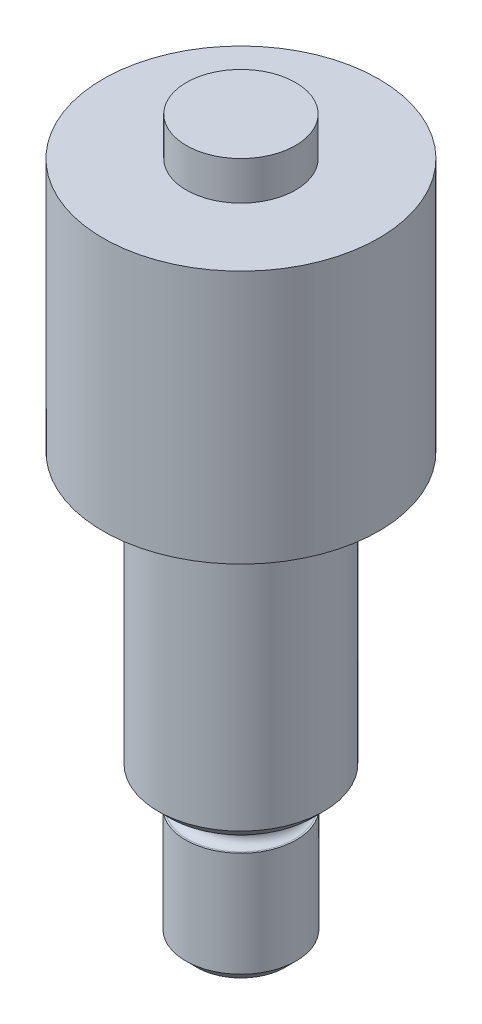
SolidWorks part; units mm, degrees
material "35"
ref_plane "前视基准面" through (0, 0, 0) normal (0, 0, 1) x (1, 0, 0)
ref_plane "上视基准面" through (0, 0, 0) normal (0, 1, 0) x (1, 0, 0)
ref_plane "右视基准面" through (0, 0, 0) normal (1, 0, 0) x (0, 0, -1)
sketch "草图1" plane through (0, 0, 0) normal (0, 0, 1) x (1, 0, 0)
  line L0 (0, 0) -> (9.9, 0)
  line L1 (9.9, 0) -> (9.9, -7)
  line L2 (9.9, -7) -> (25, -7)
  line L3 (25, -7) -> (25, -53)
  line L4 (25, -53) -> (15, -53)
  line L5 (15, -53) -> (15, -104)
  line L6 (15, -104) -> (8.2, -104)
  line L7 (8.2, -104) -> (8.2, -109)
  line L8 (8.2, -109) -> (10, -109)
  line L9 (10, -109) -> (10, -130)
  line L10 (10, -130) -> (0, -130)
  line L13 (0, -130) -> (0, 0)
  dimension "D1" = 9.9
  dimension "D2" = 7
  dimension "D3" = 46
  dimension "D4" = 5
  dimension "D5" = 130
  dimension "D7" = 25
  dimension "D8" = 15
  dimension "D9" = 8.2
  dimension "D11" = 10
  dimension "D12" = 51
revolve "旋转1" add sketch "草图1" angle 360 about L13
cosmetic thread "装饰螺纹线1" parameters "D2"=17.294
chamfer "倒角1" distance 2 angle 45 2 edges at (0, -104, -15) (0, -130, -10)
fillet "圆角1" radius 1 1 edges at (0, -53, -15)
fillet "圆角2" radius 1.5 2 edges at (0, -104, -8.2) (0, -109, -8.2)
